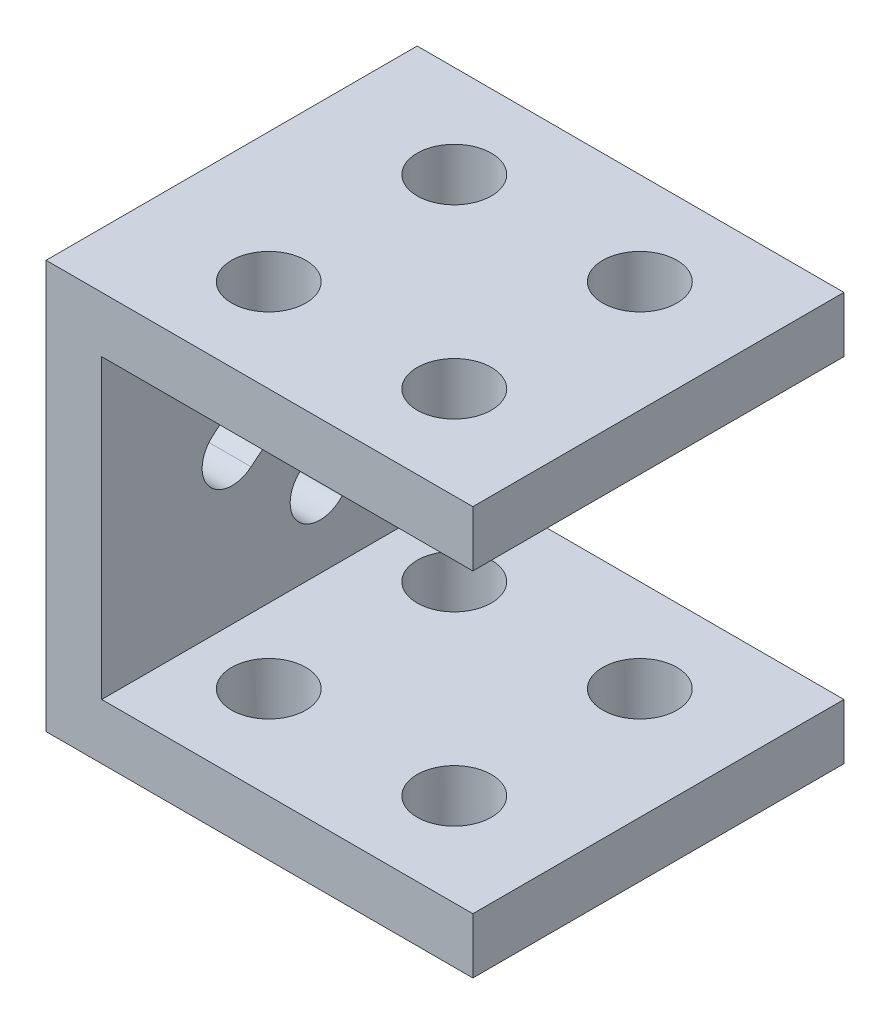
from build123d import *

# Parameters (mm, degrees)
BOSS_EXTRUDE1_DEPTH = 100
SKETCH2_R           = 10
CUT_EXTRUDE1_DEPTH  = 500
CUT_EXTRUDE2_DEPTH  = 500


with BuildPart() as part:
    # Sketch1 → Boss-Extrude1 (new body)
    with BuildSketch(Plane.XY):
        Polygon((0, 0), (100, 0), (100, -15), (-15, -15), (-15, 95), (100, 95), (100, 80), (0, 80), align=None)
    extrude(amount=BOSS_EXTRUDE1_DEPTH)

    # Sketch2 → Cut-Extrude1 (cut)
    with BuildSketch(Plane(origin=(0, 95, 0), x_dir=(1, 0, 0), z_dir=(0, 1, 0))):
        with Locations(Location((20, -25, 0), (0, 0, 270))):
            Circle(SKETCH2_R)
        with Locations(Location((70, -25, 0), (0, 0, 270))):
            Circle(SKETCH2_R)
        with Locations(Location((20, -75, 0), (0, 0, 270))):
            Circle(SKETCH2_R)
        with Locations(Location((70, -75, 0), (0, 0, 270))):
            Circle(SKETCH2_R)
    extrude(amount=-CUT_EXTRUDE1_DEPTH, mode=Mode.SUBTRACT)

    # Sketch3 → Cut-Extrude2 (cut)
    with BuildSketch(Plane(origin=(0, 0, 0), x_dir=(0, 0, -1), z_dir=(1, 0, 0))):
        with BuildLine():
            Line((-69.989356501, 46.65904216), (-50.973619408, 62.245711909))
            ThreePointArc((-50.973619408, 62.245711909), (-39.615619928, 61.120144392), (-40.741187444, 49.762144912))
            Line((-40.741187444, 49.762144912), (-59.756924537, 34.175475163))
            ThreePointArc((-59.756924537, 34.175475163), (-71.114924017, 35.30104268), (-69.989356501, 46.65904216))
        make_face()
        with BuildLine():
            Line((-47.157034179, 25.869701183), (-29.932799149, 44.934026231))
            ThreePointArc((-29.932799149, 44.934026231), (-18.599572272, 45.508702041), (-18.024896462, 34.175475163))
            Line((-18.024896462, 34.175475163), (-35.249131491, 15.111150116))
            ThreePointArc((-35.249131491, 15.111150116), (-46.582358369, 14.536474306), (-47.157034179, 25.869701183))
        make_face()
    extrude(amount=-CUT_EXTRUDE2_DEPTH, mode=Mode.SUBTRACT)


solid = part.part
